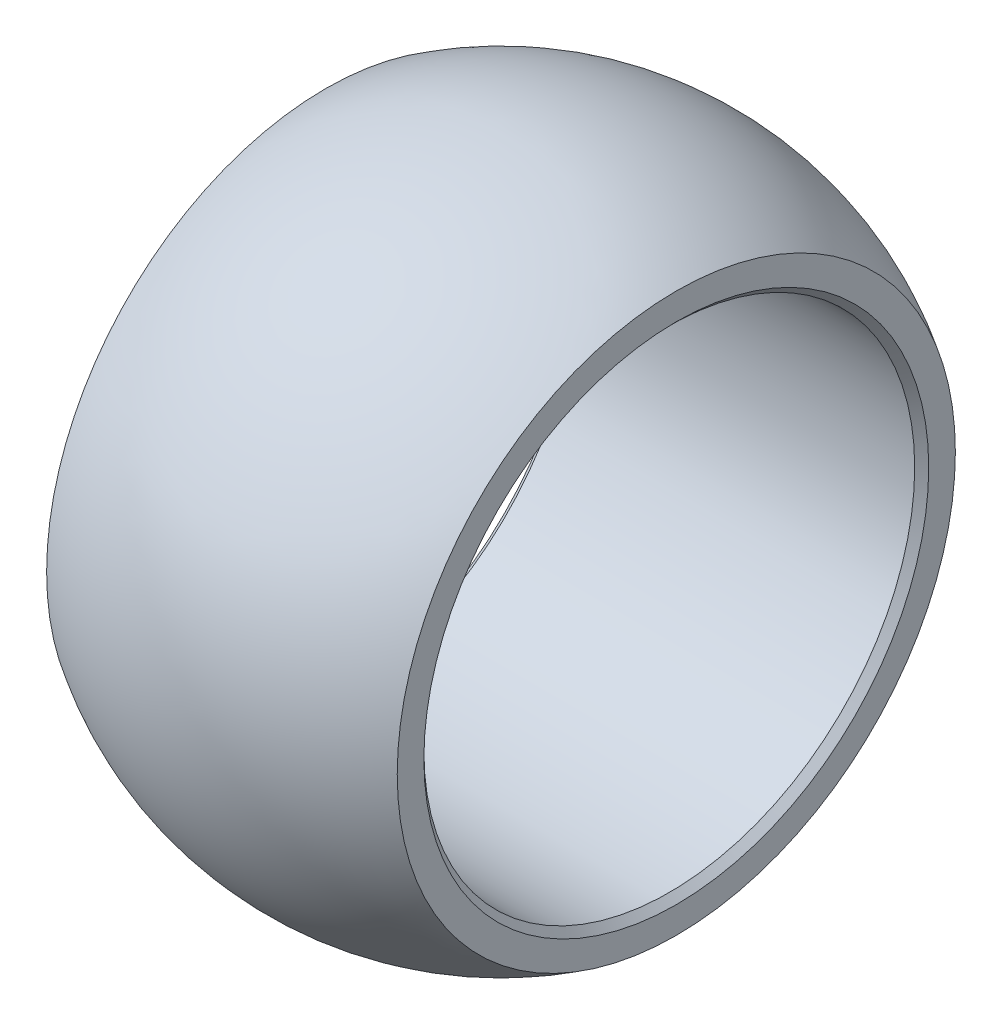
SolidWorks part; units mm, degrees
material "普通碳钢"
ref_plane "前视" through (0, 0, 0) normal (0, 0, 1) x (1, 0, 0)
ref_plane "上视" through (0, 0, 0) normal (0, 1, 0) x (1, 0, 0)
ref_plane "右视" through (0, 0, 0) normal (1, 0, 0) x (0, 0, -1)
sketch "草图1" plane through (0, 0, 0) normal (0, 0, 1) x (1, 0, 0)
  line L0 (-75.3934, 0) -> (86.8004, 0) construction
  line L1 (0, 52.0446) -> (0, -42.0635) construction
  line L2 (-12.5, 19.8997) -> (-12.5, 17.5)
  line L3 (12.5, 19.8997) -> (12.5, 17.5)
  line L4 (-12.5, 17.5) -> (12.5, 17.5)
  arc A1 (12.5, 19.8997) -> (-12.5, 19.8997) centre (0, 0) ccw
  dimension "D2" = 25
  dimension "D3" = 17.5
revolve "旋转1" add sketch "草图1" angle 360 about L0
chamfer "倒角1" distance 0.5 angle 45 2 edges at (-12.5, 0, 17.5) (12.5, 0, 17.5)
